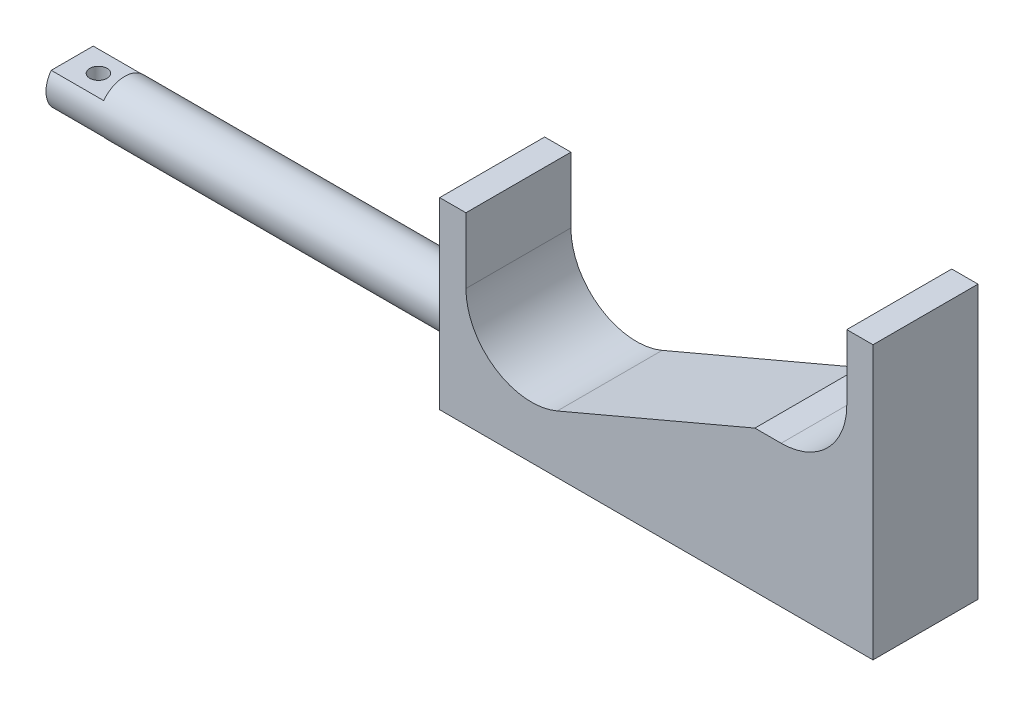
SolidWorks part; units mm, degrees
ref_plane "前视基准面" through (0, 0, 0) normal (0, 0, 1) x (1, 0, 0)
ref_plane "上视基准面" through (0, 0, 0) normal (0, 1, 0) x (1, 0, 0)
ref_plane "右视基准面" through (0, 0, 0) normal (1, 0, 0) x (0, 0, -1)
sketch "草图2" plane through (0, 0, 0) normal (0, 0, 1) x (1, 0, 0)
  line L2 (2.3432, 0.9959) -> (40, 17)
  line L4 (40, 17) -> (45, 17)
  line L6 (-15.046, 12.5) -> (-15.046, 25)
  line L7 (-15.046, 25) -> (-20.046, 25)
  line L8 (-20.046, 25) -> (-20.046, 0)
  line L9 (-20.046, 0) -> (-20.046, -10)
  line L10 (-20.046, -10) -> (40, -10)
  line L11 (40, -10) -> (57.5, -10)
  line L12 (57.5, -10) -> (62.5, -10)
  line L13 (62.5, -10) -> (62.5, 42)
  line L14 (62.5, 42) -> (57.5, 42)
  line L15 (57.5, 42) -> (57.5, 29.5)
  arc A0 (45, 17) -> (57.5, 29.5) centre (45, 29.5) ccw
  arc A1 (-15.046, 12.5) -> (2.3432, 0.9959) centre (-2.546, 12.5) ccw
extrude "凸台-拉伸1" add sketch "草图2" along normal blind 20
sketch "草图3" plane through (-20.046, 0, 0) normal (-1, 0, 0) x (0, 0, 1)
  line L0 (20, -10) -> (0, -10) construction
  circle A0 centre (10, 0) radius 5
  dimension "D1" = 10
extrude "凸台-拉伸2" add sketch "草图3" along normal blind 80
sketch "草图4" plane through (-100.046, 0, 0) normal (-1, 0, 0) x (0, 0, 1)
  line L1 (3.7839, 3) -> (15, 3)
  line L2 (3.7839, 3) -> (3.7839, -3)
  line L3 (3.7839, -3) -> (15, -3)
  line L4 (15, 3) -> (15, -3)
  dimension "D1" = 6
  dimension "D2" = 3
extrude "切除-拉伸1" cut sketch "草图4" against normal blind 10 flip side to cut
hole_wizard "M4 螺纹孔1" positions "草图7" profile "草图6" tap size "M4" standard "Iso"
sketch "草图7" plane through (0, 3, 0) normal (0, 1, 0) x (1, 0, 0)
  point P0 (-95.046, -10)
  point P4 (-95.046, -10)
sketch "草图6" plane through (-95.046, 3, 10) normal (1, 0, 0) x (0, 0, 1)
  line L0 (0, 0) -> (0, 11.0914)
  line L1 (0, 11.0914) -> (1.65, 10.1)
  line L2 (1.65, 10.1) -> (1.65, 0)
  line L5 (1.65, 0) -> (0, 0)
  line L10 (0, 11.0914) -> (-1.65, 10.1) construction
  line L11 (0, -6.35) -> (0, 107.95) construction
  dimension "螺纹孔钻头直径" = 3.3
  dimension "螺纹孔钻头深度" = 10.1
  dimension "导头角度" = 118
cosmetic thread "孔螺蚊线1" parameters "D1"=6, "D2"=4
